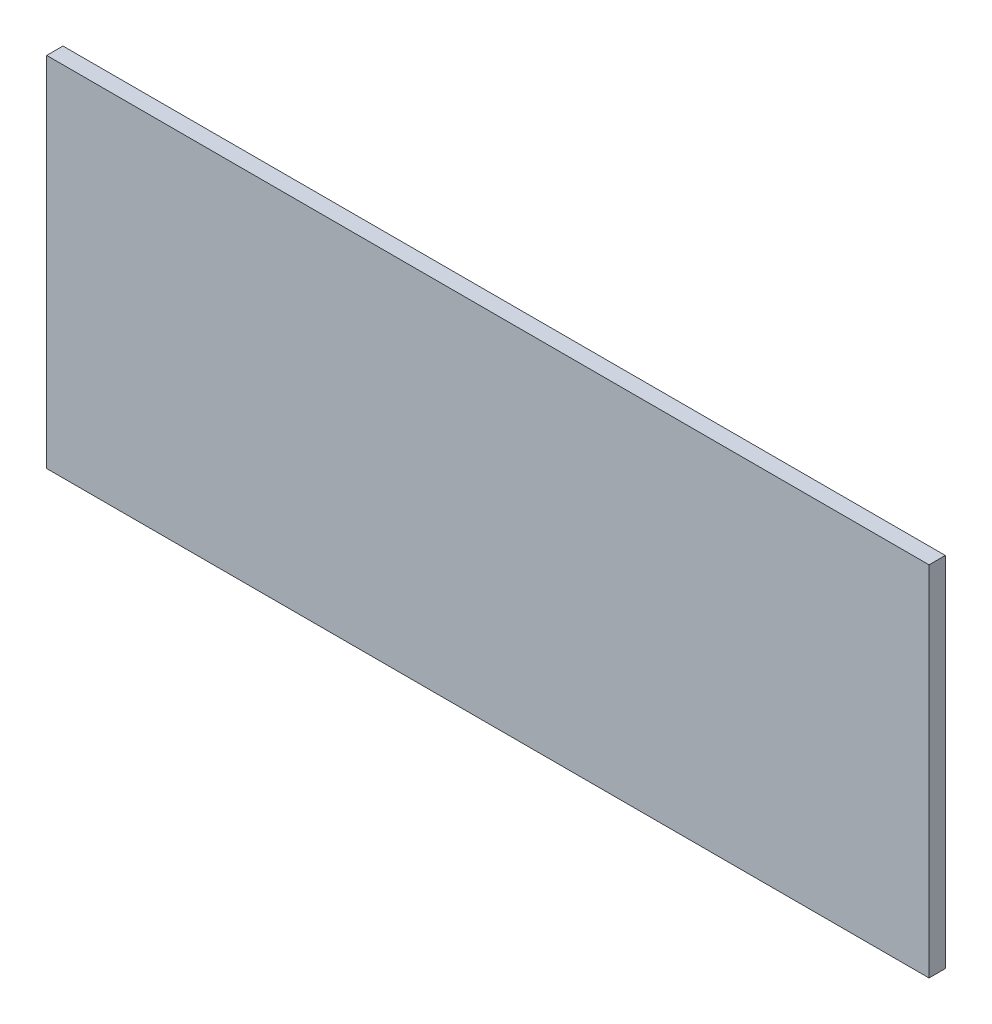
from build123d import *

# Parameters (mm, degrees)
SKETCH_1_W      = 217
SKETCH_1_H      = 88
EXTRUDE_1_DEPTH = 4


with BuildPart() as part:
    # 草图1 → 凸台-拉伸1 (new body)
    with BuildSketch(Plane.XY):
        Rectangle(SKETCH_1_W, SKETCH_1_H)
    extrude(amount=EXTRUDE_1_DEPTH)


solid = part.part
